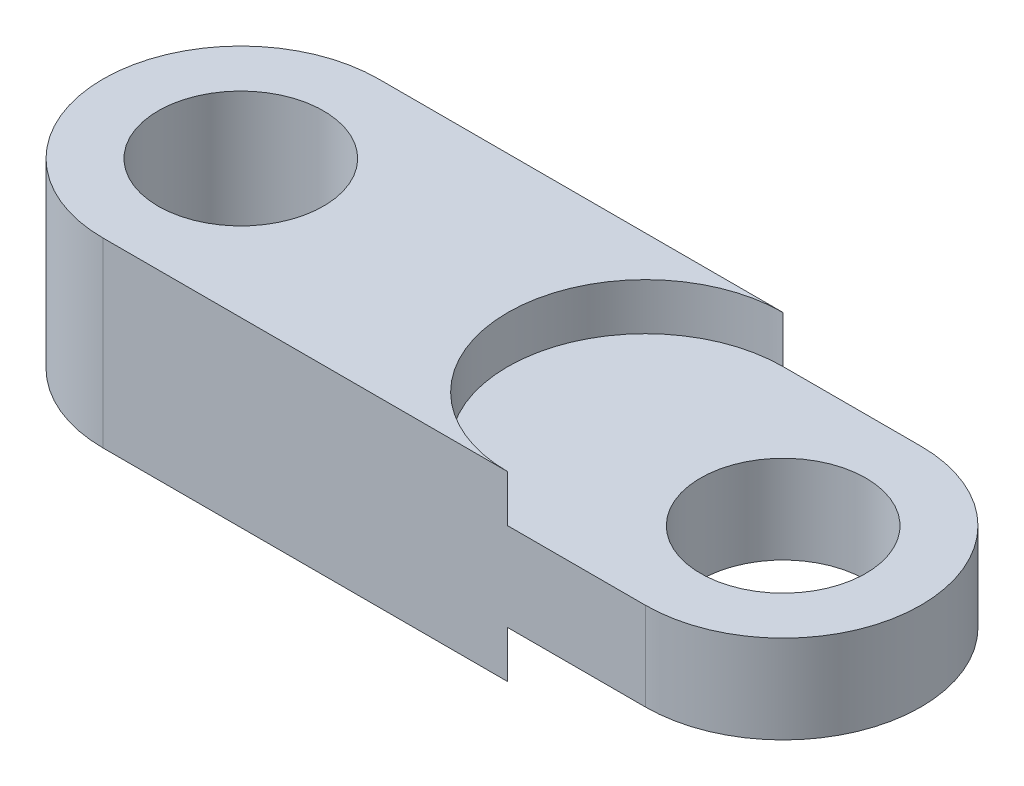
from build123d import *

# Parameters (mm, degrees)
SKETCH2_R           = 3.81
BOSS_EXTRUDE1_DEPTH = 8.382
SKETCH3_W           = 6.35
SKETCH3_H           = 2.159
CUT_EXTRUDE3_DEPTH  = 35.847818067
SKETCH4_R           = 6.35
CUT_EXTRUDE5_DEPTH  = 2.159
CUT_EXTRUDE6_START  = -2.159
SKETCH5_R           = 6.35
CUT_EXTRUDE6_DEPTH  = 2.159
SCALE1_SCALE        = 2


with BuildPart() as part:
    # Sketch2 → Boss-Extrude1 (new body)
    with BuildSketch(Plane(origin=(0, 0, 0), x_dir=(1, 0, 0), z_dir=(0, 1, 0))):
        with BuildLine():
            Line((0, 6.35), (25, 6.35))
            ThreePointArc((25, 6.35), (31.35, 0), (25, -6.35))
            Line((25, -6.35), (0, -6.35))
            ThreePointArc((0, -6.35), (-6.35, 0), (0, 6.35))
        make_face()
        with Locations(Location((0, 0, 0), (0, 0, 270))):
            Circle(SKETCH2_R, mode=Mode.SUBTRACT)
        with Locations(Location((25, 0, 0), (0, 0, 270))):
            Circle(SKETCH2_R, mode=Mode.SUBTRACT)
    extrude(amount=BOSS_EXTRUDE1_DEPTH)

    # Sketch3 → Cut-Extrude3 (cut, through all)
    with BuildSketch(Plane.XY.offset(6.35)):
        Polygon((52.142468872, 2.159), (25, 2.159), (25, 0), (54.039711746, 0), align=None)
        with Locations((21.825, 1.0795)):
            Rectangle(SKETCH3_W, SKETCH3_H)
        Polygon((49.831282098, 8.382), (25, 8.382), (25, 6.223), (51.556048347, 6.223), align=None)
        with Locations((21.825, 7.3025)):
            Rectangle(SKETCH3_W, SKETCH3_H)
    extrude(amount=-CUT_EXTRUDE3_DEPTH, mode=Mode.SUBTRACT)

    # Sketch4 → Cut-Extrude5 (cut)
    with BuildSketch(Plane.XZ):
        with Locations((18.65, 0)):
            Circle(SKETCH4_R)
    extrude(amount=-CUT_EXTRUDE5_DEPTH, mode=Mode.SUBTRACT)

    # Sketch5 → Cut-Extrude6 (cut)
    with BuildSketch(Plane(origin=(0, 8.382, 0), x_dir=(1, 0, 0), z_dir=(0, 1, 0)).offset(CUT_EXTRUDE6_START)):
        with Locations((18.65, 0)):
            Circle(SKETCH5_R)
    extrude(amount=CUT_EXTRUDE6_DEPTH, mode=Mode.SUBTRACT)


with BuildPart() as part_1:
    # Scale1: scaled about (0, 0, 0)
    add(part.part.scale(SCALE1_SCALE))


solid = part_1.part
